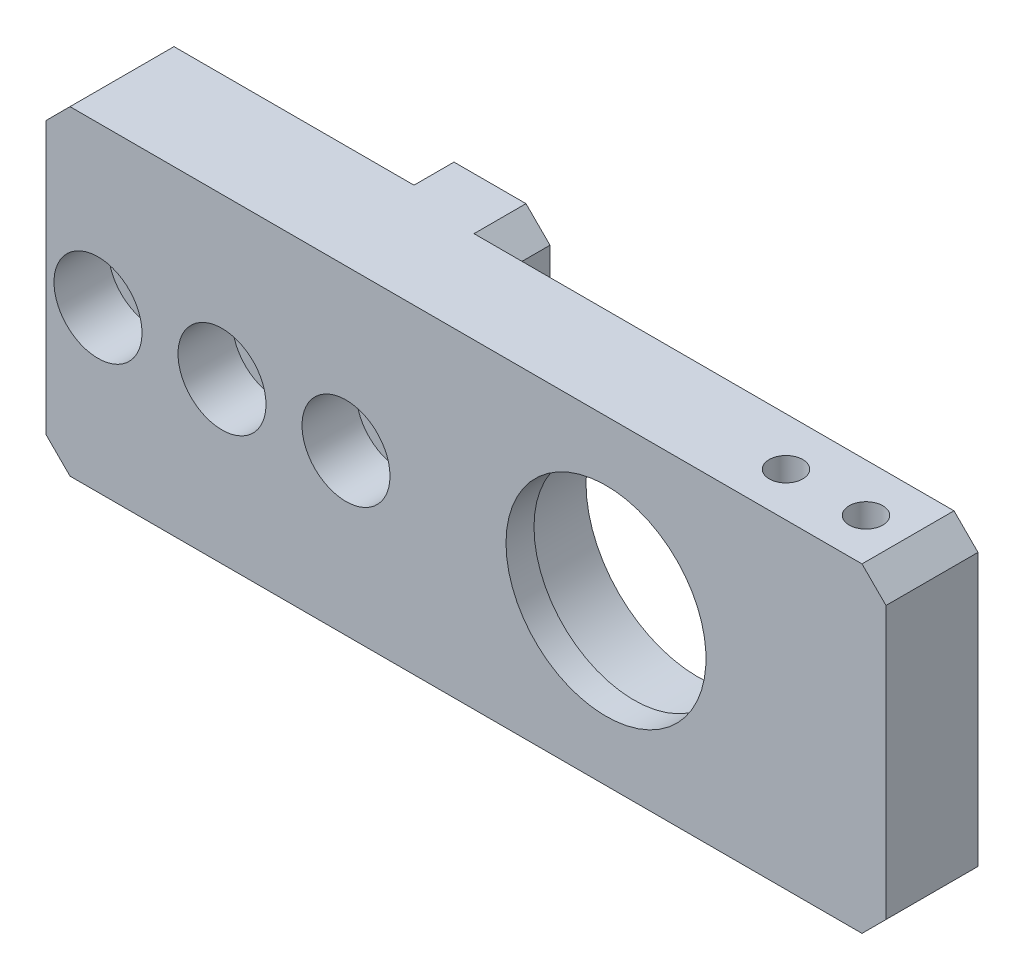
SolidWorks part; units mm, degrees
ref_plane "前视基准面" through (0, 0, 0) normal (0, 0, 1) x (1, 0, 0)
ref_plane "上视基准面" through (0, 0, 0) normal (0, 1, 0) x (1, 0, 0)
ref_plane "右视基准面" through (0, 0, 0) normal (1, 0, 0) x (0, 0, -1)
sketch "草图1" plane through (0, 0, 0) normal (0, 0, 1) x (1, 0, 0)
  line L1 (-52.5, -20) -> (52.5, -20)
  line L2 (-52.5, -20) -> (-52.5, 20)
  line L3 (-52.5, 20) -> (52.5, 20)
  line L4 (52.5, -20) -> (52.5, 20)
  line L5 (-52.5, -20) -> (52.5, 20) construction
  line L6 (-52.5, 20) -> (52.5, -20) construction
  point P0 (0, 0)
  dimension "D1" = 40
  dimension "D2" = 105
extrude "凸台-拉伸1" add sketch "草图1" along normal blind 18
sketch "草图2" plane through (0, 0, 0) normal (0, 0, -1) x (-1, 0, 0)
  line L0 (52.5, -20) -> (-52.5, -20) construction
  line L1 (52.5, 20) -> (22.5, 20)
  line L2 (52.5, 20) -> (52.5, -20)
  line L3 (52.5, -20) -> (22.5, -20)
  line L4 (22.5, 20) -> (22.5, -20)
  dimension "D1" = 30
extrude "切除-拉伸1" cut sketch "草图2" against normal blind 5
sketch "草图3" plane through (0, 0, 0) normal (0, 0, -1) x (-1, 0, 0)
  line L0 (22.5, -20) -> (-52.5, -20) construction
  line L1 (-52.5, 20) -> (7.5, 20)
  line L2 (-52.5, 20) -> (-52.5, -20)
  line L3 (-52.5, -20) -> (7.5, -20)
  line L4 (7.5, 20) -> (7.5, -20)
  dimension "D1" = 60
extrude "切除-拉伸2" cut sketch "草图3" against normal blind 6.5
hole_wizard "打孔尺寸(%根据)内六角圆柱头螺钉的类型1" positions "草图4" profile "草图5" counterbore size "M6" standard "GB" end condition through all
sketch "草图4" plane through (0, 0, 18) normal (0, 0, 1) x (1, 0, 0)
  line L0 (0, 0) -> (-15, 0) construction
  line L1 (-52.5, 20) -> (-52.5, -20) construction
  point P0 (-46, 0)
  point P2 (-30.5, 0)
  point P4 (-15, 0)
  point P10 (0, 0)
  dimension "D1" = 37.5
  dimension "D2" = 15.5
  dimension "D3" = 15.5
sketch "草图5" plane through (-46, 0, 18) normal (1, 0, 0) x (0, -1, 0)
  line L0 (0, 0) -> (0, 18)
  line L1 (0, 18) -> (3.3, 18)
  line L3 (3.3, 18) -> (3.3, 6.8)
  line L4 (3.3, 6.8) -> (5.5, 6.8)
  line L5 (5.5, 6.8) -> (5.5, 0)
  line L7 (5.5, 0) -> (0, 0)
  line L11 (0, -6.35) -> (0, 107.95) construction
  dimension "通孔孔直径" = 6.6
  dimension "通孔孔深度" = 18
  dimension "柱形沉头孔直径" = 11
  dimension "柱形沉头孔深度" = 6.8
sketch "草图6" plane through (0, 0, 0) normal (0, 0, -1) x (-1, 0, 0)
  circle A0 centre (15, 0) radius 5
  dimension "D1" = 10
extrude "切除-拉伸3" cut sketch "草图6" against normal blind 2
sketch "草图7" plane through (0, 0, 6.5) normal (0, 0, -1) x (-1, 0, 0)
  line L0 (0, 0) -> (-17.5, 0) construction
  line L1 (-52.5, 20) -> (-52.5, -20) construction
  circle A0 centre (-17.5, 0) radius 14
  point P5 (0, 0)
  dimension "D1" = 28
  dimension "D2" = 35
extrude "切除-拉伸4" cut sketch "草图7" against normal blind 8
sketch "草图8" plane through (0, 0, 14.5) normal (0, 0, -1) x (-1, 0, 0)
  circle A0 centre (-17.5, 0) radius 12.5
  dimension "D1" = 25
extrude "切除-拉伸5" cut sketch "草图8" against normal through all
chamfer "倒角1" distance 3 angle 45 8 edges at (-22.5, -20, 2.5) (-7.5, -20, 3.25) (-7.5, 20, 3.25) (-22.5, 20, 2.5) (-52.5, 20, 11.5) (-52.5, -20, 11.5) (52.5, -20, 12.25) (52.5, 20, 12.25)
hole_wizard "M5 螺纹孔1" positions "草图9" profile "草图10" tap size "M5" standard "GB"
sketch "草图9" plane through (0, -20, 0) normal (0, -1, 0) x (-1, 0, 0)
  line L6 (49.5, -18) -> (-49.5, -18) construction
  line L7 (-52.5, -18) -> (-52.5, -6.5) construction
  point P0 (-44.5, -12.5)
  point P2 (-34.5, -12.5)
  point P18 (0, 0)
  dimension "D1" = 5.5
  dimension "D2" = 8
  dimension "D3" = 10
sketch "草图10" plane through (44.5, -20, 12.5) normal (1, 0, 0) x (0, 0, -1)
  line L0 (0, 0) -> (0, 13.6618)
  line L1 (0, 13.6618) -> (2.1, 12.4)
  line L2 (2.1, 12.4) -> (2.1, 0)
  line L5 (2.1, 0) -> (0, 0)
  line L10 (0, 13.6618) -> (-2.1, 12.4) construction
  line L11 (0, -6.35) -> (0, 107.95) construction
  dimension "螺纹孔钻头直径" = 4.2
  dimension "螺纹孔钻头深度" = 12.4
  dimension "导头角度" = 118
cosmetic thread "孔螺蚊线1" parameters "D1"=10, "D2"=5
cosmetic thread "孔螺蚊线2" parameters "D1"=10, "D2"=5
mirror "镜向1" about plane through (0, 0, 0) normal (0, 1, 0) of "M5 螺纹孔1"
